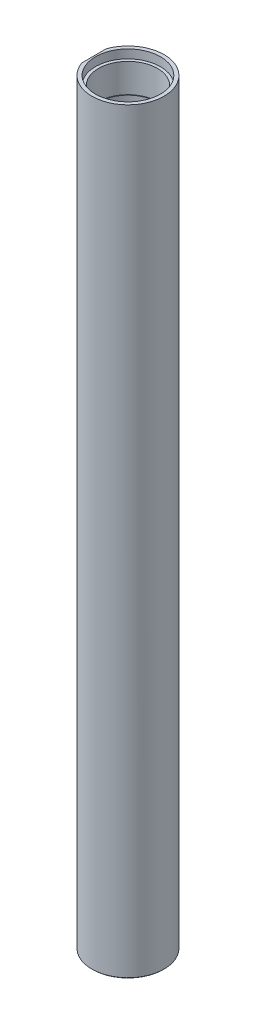
from build123d import *

# Parameters (mm, degrees)
SKETCH1_R                = 50
SKETCH1_R_2              = 40
BOSS_EXTRUDE1_DEPTH      = 1049
SKETCH10_R               = 45
CUT_EXTRUDE8_DEPTH       = 12
SKETCH13_R               = 44.375
CUT_EXTRUDE10_DEPTH      = 40
CHAMFER5_SIZE            = 1
SKETCH14_R               = 40.875
CUT_EXTRUDE11_DEPTH      = 40
CUT_EXTRUDE12_DEPTH      = 1052.380521029
CUT_EXTRUDE12_DEPTH_BACK = 1052.380521029
SKETCH15_W               = 6
SKETCH15_H               = 40


with BuildPart() as part:
    # Sketch1 → Boss-Extrude1 (new body)
    with BuildSketch(Plane(origin=(0, 0, 0), x_dir=(1, 0, 0), z_dir=(0, 1, 0))):
        with Locations(Location((0, 0, 0), (0, 0, 270))):
            Circle(SKETCH1_R)
        with Locations(Location((0, 0, 0), (0, 0, 270))):
            Circle(SKETCH1_R_2, mode=Mode.SUBTRACT)
    extrude(amount=BOSS_EXTRUDE1_DEPTH)

    # Sketch10 → Cut-Extrude8 (cut)
    with BuildSketch(Plane(origin=(0, 1049, 0), x_dir=(1, 0, 0), z_dir=(0, 1, 0))):
        with Locations(Location((0, 0, 0), (0, 0, 270))):
            Circle(SKETCH10_R)
    extrude(amount=-CUT_EXTRUDE8_DEPTH, mode=Mode.SUBTRACT)

    # Sketch13 → Cut-Extrude10 (cut)
    with BuildSketch(Plane.XZ):
        with Locations(Location((0, 0, 0), (0, 0, 270))):
            Circle(SKETCH13_R)
    extrude(amount=-CUT_EXTRUDE10_DEPTH, mode=Mode.SUBTRACT)

    # Chamfer5
    chamfer5_edges = [part.edges().sort_by_distance(p)[0] for p in [
        (0, 0, 44.375),
        (0, 0, -50),
    ]]
    chamfer(chamfer5_edges, length=CHAMFER5_SIZE)

    # Sketch14 → Cut-Extrude11 (cut)
    with BuildSketch(Plane(origin=(0, 1037, 0), x_dir=(1, 0, 0), z_dir=(0, 1, 0))):
        with Locations(Location((0, 0, 0), (0, 0, 270))):
            Circle(SKETCH14_R)
    extrude(amount=-CUT_EXTRUDE11_DEPTH, mode=Mode.SUBTRACT)

    # Sketch15 → Cut-Extrude12 (cut, two sides: drawn at the far end of the back side and taken through both)
    with BuildSketch(Plane.XY.offset(-CUT_EXTRUDE12_DEPTH_BACK)):
        with Locations((-50, 1049)):
            Rectangle(SKETCH15_W, SKETCH15_H)
    extrude(amount=CUT_EXTRUDE12_DEPTH + CUT_EXTRUDE12_DEPTH_BACK, mode=Mode.SUBTRACT)


solid = part.part
